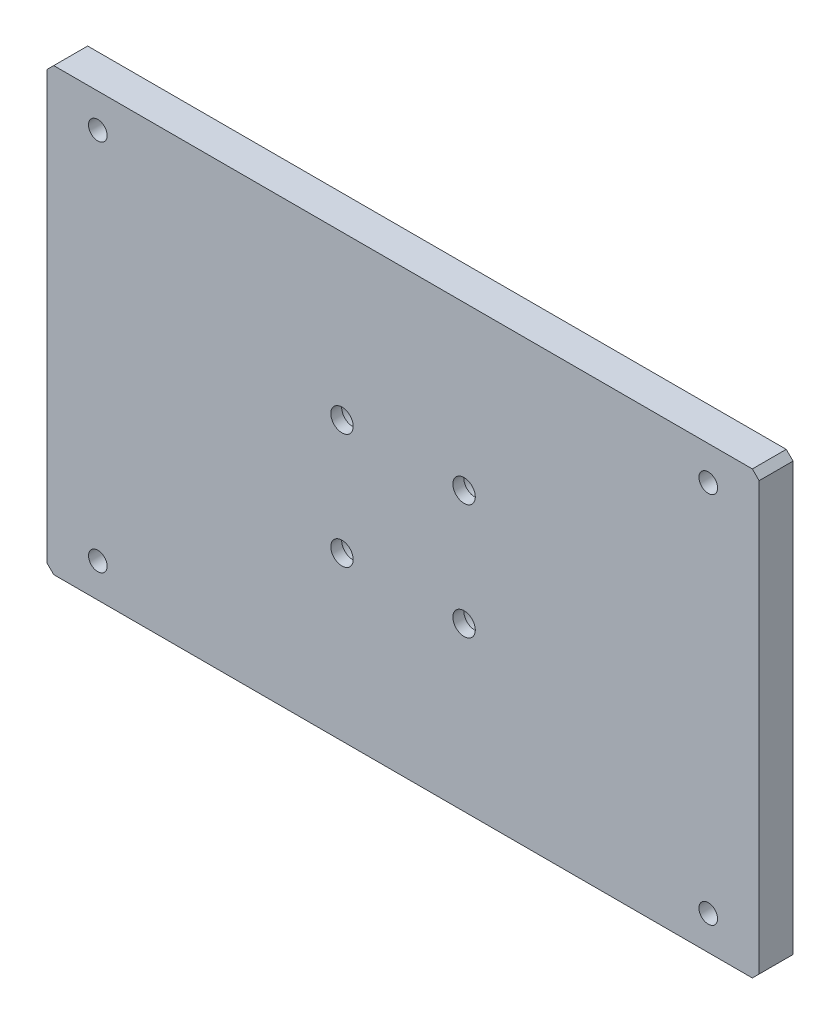
from build123d import *

# Parameters (mm, degrees)
SKETCH1_W                                           = 210
SKETCH1_H                                           = 130
BOSS_EXTRUDE1_DEPTH                                 = 10
HOLE_SIZE_PER_SOCKET_HEAD_CAP_SCREW_TYP_D           = 6.6
HOLE_SIZE_PER_SOCKET_HEAD_CAP_SCREW_TYP_CBORE_D     = 11
HOLE_SIZE_PER_SOCKET_HEAD_CAP_SCREW_TYP_CBORE_DEPTH = 6.8
HOLE_SIZE_PER_SOCKET_HEAD_CAP_SCREW_2_D             = 5.5
HOLE_SIZE_PER_SOCKET_HEAD_CAP_SCREW_2_CBORE_D       = 10
HOLE_SIZE_PER_SOCKET_HEAD_CAP_SCREW_2_CBORE_DEPTH   = 5.7
CHAMFER1_SIZE                                       = 2


with BuildPart() as part:
    # Sketch1 → Boss-Extrude1 (new body)
    with BuildSketch(Plane.XY):
        Rectangle(SKETCH1_W, SKETCH1_H)
    extrude(amount=BOSS_EXTRUDE1_DEPTH)

    # Hole size _per socket head cap screw typ (through all)
    with Locations(Plane(origin=(-18, -17, 0), x_dir=(-1, 0, 0), z_dir=(0, 0, -1))):
        with Locations((0, 0), (-36, 0), (-36, 34), (0, 34)):
            CounterBoreHole(HOLE_SIZE_PER_SOCKET_HEAD_CAP_SCREW_TYP_D / 2, HOLE_SIZE_PER_SOCKET_HEAD_CAP_SCREW_TYP_CBORE_D / 2, HOLE_SIZE_PER_SOCKET_HEAD_CAP_SCREW_TYP_CBORE_DEPTH)

    # Hole size _per socket head cap screw 2 (through all)
    with Locations(Plane(origin=(-90, -55, 0), x_dir=(-1, 0, 0), z_dir=(0, 0, -1))):
        with Locations((0, 0), (0, 110), (-180, 110), (-180, 0)):
            CounterBoreHole(HOLE_SIZE_PER_SOCKET_HEAD_CAP_SCREW_2_D / 2, HOLE_SIZE_PER_SOCKET_HEAD_CAP_SCREW_2_CBORE_D / 2, HOLE_SIZE_PER_SOCKET_HEAD_CAP_SCREW_2_CBORE_DEPTH)

    # Chamfer1
    chamfer1_edges = [part.edges().sort_by_distance(p)[0] for p in [
        (105, -65, 5),
        (-105, -65, 5),
        (-105, 65, 5),
        (105, 65, 5),
    ]]
    chamfer(chamfer1_edges, length=CHAMFER1_SIZE)


solid = part.part
